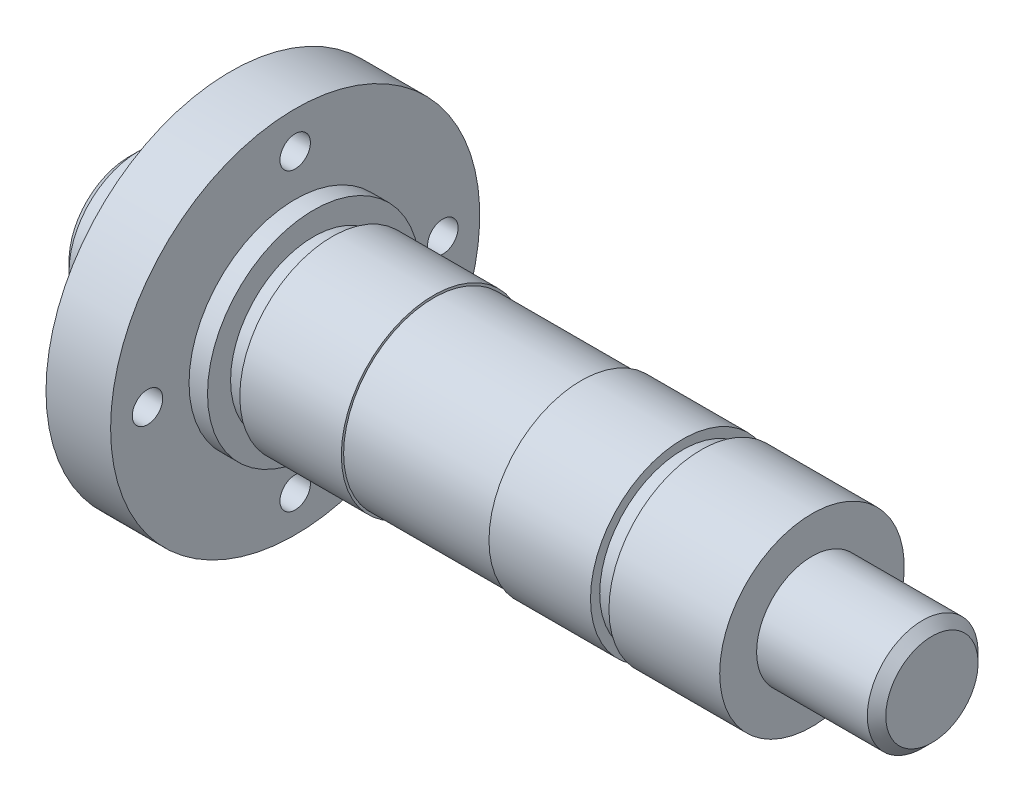
SolidWorks part; units mm, degrees
ref_plane "Front" through (0, 0, 0) normal (0, 0, 1) x (1, 0, 0)
ref_plane "Top" through (0, 0, 0) normal (0, 1, 0) x (1, 0, 0)
ref_plane "Right" through (0, 0, 0) normal (1, 0, 0) x (0, 0, -1)
sketch "Sketch1" plane through (0, 0, 0) normal (0, 0, 1) x (1, 0, 0)
  line L0 (0, 0) -> (87, 0)
  line L1 (0, 0) -> (0, 7.5)
  line L2 (0, 7.5) -> (8, 7.5)
  line L3 (8, 7.5) -> (8, 10)
  line L4 (8, 10) -> (11, 10)
  line L5 (11, 10) -> (11, 20)
  line L6 (11, 20) -> (18, 20)
  line L7 (18, 20) -> (18, 11.5)
  line L8 (18, 11.5) -> (20, 11.5)
  line L9 (20, 11.5) -> (20, 10)
  line L10 (20, 10) -> (33, 10)
  line L11 (33, 10) -> (33, 9.75)
  line L12 (33, 9.75) -> (49, 9.75)
  line L13 (49, 9.75) -> (49, 10)
  line L14 (49, 10) -> (60, 10)
  line L15 (60, 10) -> (60, 9)
  line L16 (60, 9) -> (62, 9)
  line L17 (62, 9) -> (62, 10)
  line L18 (62, 10) -> (74, 10)
  line L19 (74, 10) -> (74, 6)
  line L20 (74, 6) -> (87, 6)
  line L21 (87, 6) -> (87, 0)
  line L22 (0, 0) -> (117.8358, 0) construction
  dimension "D1" = 15
  dimension "D2" = 20
  dimension "D3" = 40
  dimension "D4" = 23
  dimension "D5" = 20
  dimension "D6" = 19.5
  dimension "D7" = 20
  dimension "D8" = 18
  dimension "D9" = 20
  dimension "D10" = 12
  dimension "D11" = 8
  dimension "D12" = 3
  dimension "D13" = 7
  dimension "D14" = 2
  dimension "D15" = 13
  dimension "D16" = 16
  dimension "D17" = 11
  dimension "D18" = 2
  dimension "D19" = 12
  dimension "D20" = 87
revolve "Revolve1" add sketch "Sketch1" angle 360 about L22
cosmetic thread "Cosmetic Thread1" parameters "D2"=19
hole_wizard "M6 Tapped Hole1" positions "Sketch3" profile "Sketch2" tap size "M6" standard "GB"
sketch "Sketch3" plane through (0, 0, 0) normal (-1, 0, 0) x (0, 0, 1)
  point P0 (0, 0)
sketch "Sketch2" plane through (0, 0, 0) normal (0, 1, 0) x (0, 0, 1)
  line L0 (0, 0) -> (0, 19.5022)
  line L1 (0, 19.5022) -> (2.5, 18)
  line L2 (2.5, 18) -> (2.5, 0)
  line L5 (2.5, 0) -> (0, 0)
  line L10 (0, 19.5022) -> (-2.5, 18) construction
  line L11 (0, -6.35) -> (0, 107.95) construction
  dimension "螺纹孔钻头直径" = 5
  dimension "螺纹孔钻头深度" = 18
  dimension "导头角度" = 118
cosmetic thread "孔螺蚊线1" parameters "D1"=15, "D2"=6
hole_wizard "M4 Tapped Hole1" positions "Sketch5" profile "Sketch4" tap size "M4" standard "GB" end condition through all
sketch "Sketch5" plane through (11, 0, 0) normal (-1, 0, 0) x (0, 0, 1)
  circle A0 centre (0, 0) radius 16 construction
  point P0 (0, 16)
  point P1 (-16, 0)
  point P3 (0, -16)
  point P5 (16, 0)
  dimension "D1" = 32
sketch "Sketch4" plane through (11, 16, 0) normal (0, 1, 0) x (0, 0, 1)
  line L0 (0, 0) -> (0, 76)
  line L1 (0, 76) -> (1.65, 76)
  line L2 (1.65, 76) -> (1.65, 0)
  line L5 (1.65, 0) -> (0, 0)
  line L11 (0, -6.35) -> (0, 107.95) construction
  dimension "通孔螺纹孔钻头直径" = 3.3
  dimension "通孔螺纹孔钻头深度" = 76
cosmetic thread "Cosmetic Thread2" parameters "D2"=4
cosmetic thread "Cosmetic Thread3" parameters "D2"=4
cosmetic thread "Cosmetic Thread4" parameters "D2"=4
cosmetic thread "Cosmetic Thread5" parameters "D2"=4
sketch "Sketch6" plane through (0, 0, 0) normal (0, 0, 1) x (1, 0, 0)
  line L0 (0, 0) -> (87, 0) construction
  line L1 (87, -6) -> (87, 6) construction
  line L2 (20, -11.5) -> (20, 11.5) construction
  line L3 (20, 10) -> (22, 10)
  line L4 (20, 10) -> (20, 9)
  line L5 (20, 9) -> (22, 9)
  line L6 (22, 10) -> (22, 9)
  line L7 (33, 10) -> (20, 10) construction
  dimension "D1" = 2
  dimension "D2" = 1
revolve "Cut-Revolve1" cut sketch "Sketch6" angle 360 about L0
chamfer "Chamfer1" distance 1 angle 45 2 edges at (87, 0, 6) (0, 0, 7.5)
